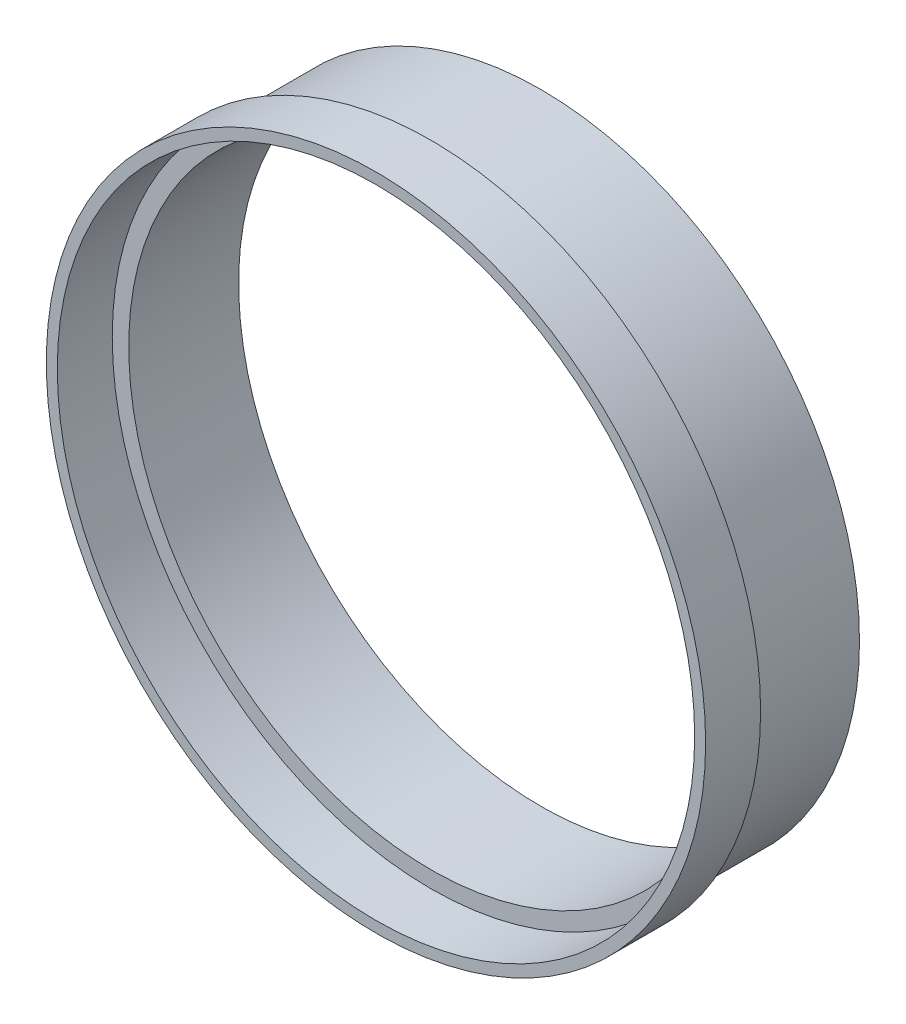
SolidWorks part; units mm, degrees
ref_plane "Front Plane" through (0, 0, 0) normal (0, 0, 1) x (1, 0, 0)
ref_plane "Top Plane" through (0, 0, 0) normal (0, 1, 0) x (1, 0, 0)
ref_plane "Right Plane" through (0, 0, 0) normal (1, 0, 0) x (0, 0, -1)
sketch "Sketch1" plane through (0, 0, 0) normal (0, 0, 1) x (1, 0, 0)
  circle A0 centre (0, 0) radius 58
  circle A1 centre (0, 0) radius 55
  dimension "D1" = 110
  dimension "D2" = 116
extrude "Boss-Extrude1" add sketch "Sketch1" along normal blind 20
sketch "Sketch2" plane through (0, 0, 20) normal (0, 0, 1) x (1, 0, 0)
  circle A0 centre (0, 0) radius 58
  circle A1 centre (0, 0) radius 60
extrude "Boss-Extrude2" add sketch "Sketch2" along normal blind 10 separate body
